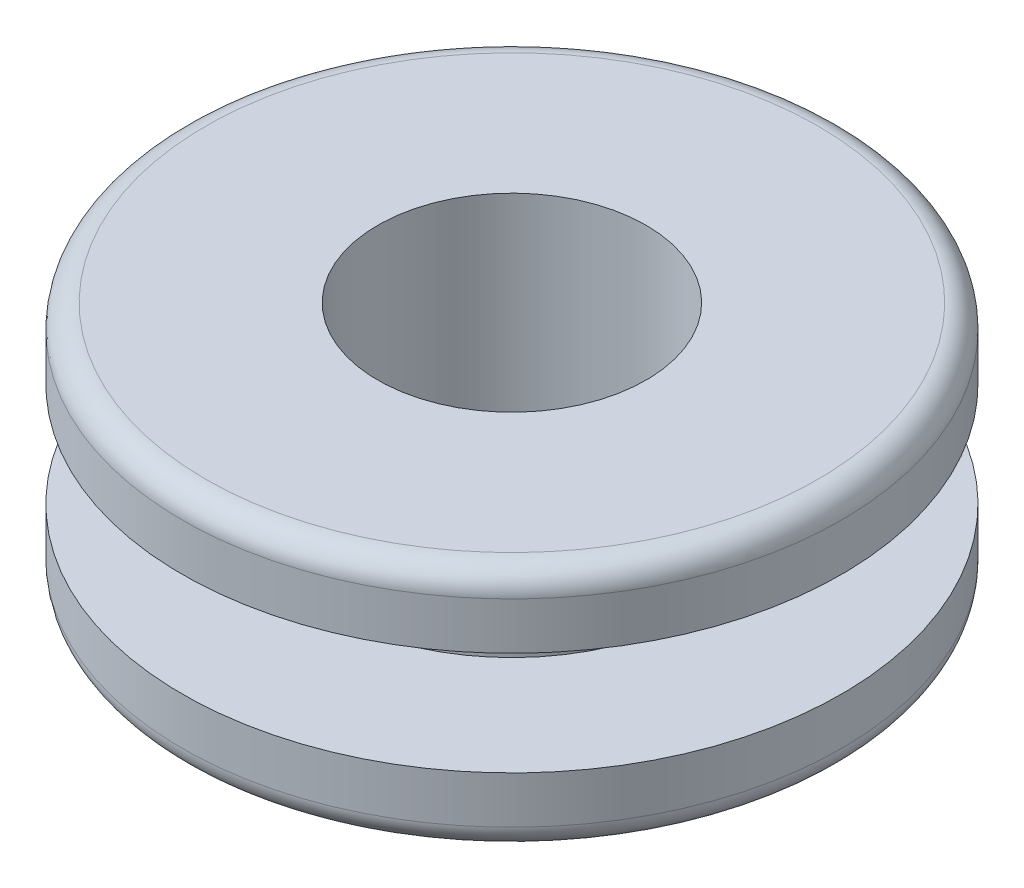
SolidWorks part; units mm, degrees
ref_plane "前视基准面" through (0, 0, 0) normal (0, 0, 1) x (1, 0, 0)
ref_plane "上视基准面" through (0, 0, 0) normal (0, 1, 0) x (1, 0, 0)
ref_plane "右视基准面" through (0, 0, 0) normal (1, 0, 0) x (0, 0, -1)
other "Configuration Table"
sketch "草图1" plane through (0, 0, 0) normal (0, 0, 1) x (1, 0, 0)
  line L0 (0, 0) -> (0, 22.457) construction
  line L1 (2.85, 5.2) -> (6.5, 5.2)
  line L2 (7, 4.7) -> (7, 3.7)
  line L3 (7, 3.7) -> (4, 3.7)
  line L4 (4, 3.7) -> (4, 1.5)
  line L5 (4, 1.5) -> (7, 1.5)
  line L6 (7, 1.5) -> (7, 0.5)
  line L7 (6.5, 0) -> (2.85, 0)
  line L8 (2.85, 0) -> (2.85, 5.2)
  arc A0 (7, 0.5) -> (6.5, 0) centre (6.5, 0.5) cw
  arc A1 (6.5, 5.2) -> (7, 4.7) centre (6.5, 4.7) cw
  point P15 (7, 5.2)
  dimension "D7" = 0.5
  dimension "D1" = 2.85
  dimension "D2" = 7
  dimension "D3" = 2.2
  dimension "D4" = 5.2
  dimension "D6" = 4
revolve "旋转1" add sketch "草图1" angle 360 about L0
